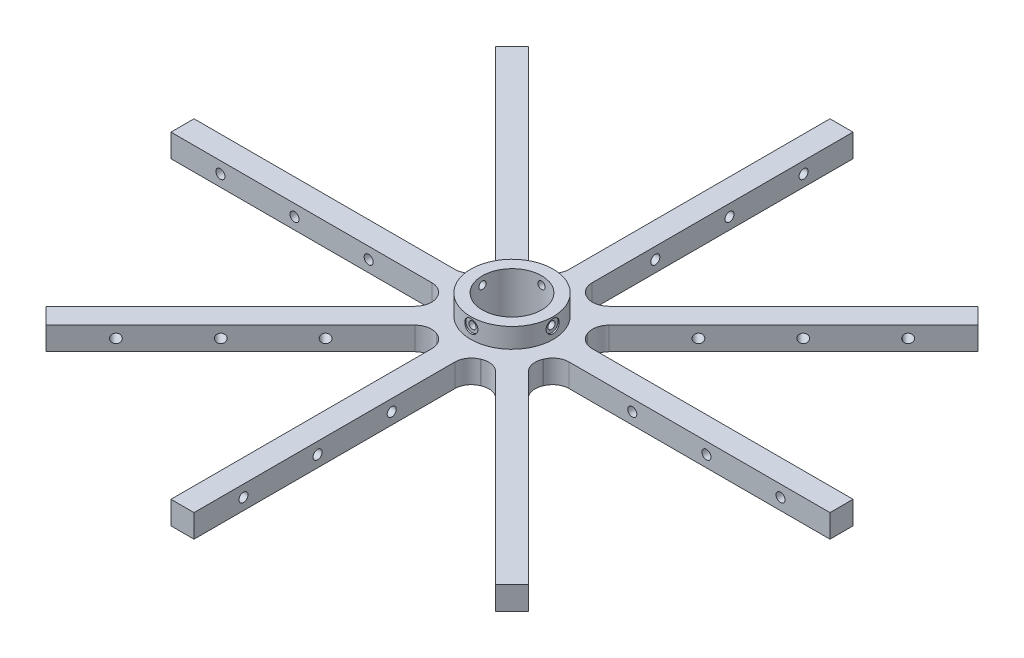
from build123d import *
from build123d.topology import SkipClean

# Parameters (mm, degrees)
SKETCH_3_R               = 25
SKETCH_3_R_2             = 18
EXTRUDE_4_DEPTH          = 7
SKETCH_4_W               = 176
SKETCH_4_H               = 14
EXTRUDE_5_DEPTH          = 7
SKETCH_5_R               = 2.75
CUT_EXTRUDE_1_DEPTH      = 14
PATTERN_CIRCULAR_1_COUNT = 8
EXTRUDE_START            = 12
SKETCH_6_R               = 25
SKETCH_6_R_2             = 18
EXTRUDE_6_DEPTH          = 12
SKETCH_7_R               = 2.2
CUT_EXTRUDE_2_DEPTH      = 43
CUT_EXTRUDE_START        = -24
SKETCH_8_R               = 4
CUT_EXTRUDE_4_DEPTH      = 43
PATTERN_CIRCULAR_2_COUNT = 4
SKETCH_10_R              = 35
SKETCH_10_R_2            = 25
EXTRUDE_7_DEPTH          = 14
FILLET_2_R               = 10


with BuildPart() as part:
    # 草图3 → 凸台-拉伸4 (new, symmetric)
    with BuildSketch(Plane(origin=(0, 0, 0), x_dir=(1, 0, 0), z_dir=(0, 1, 0))):
        with Locations(Location((0, 0, 0), (0, 0, 270))):
            Circle(SKETCH_3_R)
        with Locations(Location((0, 0, 0), (0, 0, 270))):
            Circle(SKETCH_3_R_2, mode=Mode.SUBTRACT)
    extrude(amount=EXTRUDE_4_DEPTH, both=True)

    # 草图4 → 凸台-拉伸5 (add, symmetric)
    with BuildSketch(Plane(origin=(0, 0, 0), x_dir=(1, 0, 0), z_dir=(0, 1, 0))):
        with Locations((112, 0)):
            Rectangle(SKETCH_4_W, SKETCH_4_H)
    extrude_5 = extrude(amount=EXTRUDE_5_DEPTH, both=True)

    # 草图5 → 切除-拉伸1 (cut)
    with BuildSketch(Plane.XY.offset(7)):
        with Locations((80, 0)):
            Circle(SKETCH_5_R)
        with Locations((125, 0)):
            Circle(SKETCH_5_R)
        with Locations((170, 0)):
            Circle(SKETCH_5_R)
    cut_extrude_1 = extrude(amount=-CUT_EXTRUDE_1_DEPTH, mode=Mode.SUBTRACT)

    # 阵列(圆周)1: 凸台-拉伸5, 切除-拉伸1 ×8 about axis
    pattern_circular_1_axis = Axis((0, 0, 0), (0, 1, 0))
    add([extrude_5.rotate(pattern_circular_1_axis, i * 360 / PATTERN_CIRCULAR_1_COUNT) for i in range(1, PATTERN_CIRCULAR_1_COUNT)])
    add([cut_extrude_1.rotate(pattern_circular_1_axis, i * 360 / PATTERN_CIRCULAR_1_COUNT) for i in range(1, PATTERN_CIRCULAR_1_COUNT)], mode=Mode.SUBTRACT)

    # 草图6 → 凸台-拉伸6 (add)
    with SkipClean():  # the faces are left unmerged after this step: merging them gives an invalid solid
        with BuildSketch(Plane(origin=(0, 7, 0), x_dir=(1, 0, 0), z_dir=(0, 1, 0)).offset(EXTRUDE_START)):
            with Locations(Location((0, 0, 0), (0, 0, 106.260204708))):
                Circle(SKETCH_6_R)
            with Locations(Location((0, 0, 0), (0, 0, 270))):
                Circle(SKETCH_6_R_2, mode=Mode.SUBTRACT)
        extrude(amount=-EXTRUDE_6_DEPTH)

    # 草图7 → 切除-拉伸2 (cut)
    with SkipClean():  # the faces are left unmerged after this step: merging them gives an invalid solid
        with BuildSketch(Plane.XY):
            with Locations(Location((0, 14, 0), (0, 0, 90))):
                Circle(SKETCH_7_R)
        cut_extrude_2 = extrude(amount=-CUT_EXTRUDE_2_DEPTH, mode=Mode.SUBTRACT)

    # 草图8 → 切除-拉伸4 (cut)
    with SkipClean():  # the faces are left unmerged after this step: merging them gives an invalid solid
        with BuildSketch(Plane.XY.offset(CUT_EXTRUDE_START)):
            with Locations((0, 14)):
                Circle(SKETCH_8_R)
        cut_extrude_4 = extrude(amount=-CUT_EXTRUDE_4_DEPTH, mode=Mode.SUBTRACT)

    # 阵列(圆周)2: 切除-拉伸2, 切除-拉伸4 ×4 about axis
    with SkipClean():  # the faces are left unmerged after this step: merging them gives an invalid solid
        pattern_circular_2_axis = Axis((0, 0, 0), (0, 1, 0))
        add([cut_extrude_2.rotate(pattern_circular_2_axis, i * 360 / PATTERN_CIRCULAR_2_COUNT) for i in range(1, PATTERN_CIRCULAR_2_COUNT)], mode=Mode.SUBTRACT)
        add([cut_extrude_4.rotate(pattern_circular_2_axis, i * 360 / PATTERN_CIRCULAR_2_COUNT) for i in range(1, PATTERN_CIRCULAR_2_COUNT)], mode=Mode.SUBTRACT)

    # 草图10 → 凸台-拉伸7 (add)
    with BuildSketch(Plane(origin=(0, 7, 0), x_dir=(1, 0, 0), z_dir=(0, 1, 0))):
        Circle(SKETCH_10_R)
        with Locations(Location((0, 0, 0), (0, 0, 270))):
            Circle(SKETCH_10_R_2, mode=Mode.SUBTRACT)
    extrude(amount=-EXTRUDE_7_DEPTH)

    # 圆角2
    fillet_2_edges = [part.edges().sort_by_distance(p)[0] for p in [
        (19.298963838, 0, -29.198458774),
        (34.292856399, 0, 7),
        (34.292856399, 0, -7),
        (19.298963838, 0, 29.198458774),
        (29.198458774, 0, 19.298963838),
        (-7, 0, 34.292856399),
        (7, 0, 34.292856399),
        (-29.198458774, 0, 19.298963838),
        (-19.298963838, 0, 29.198458774),
        (-34.292856399, 0, -7),
        (-34.292856399, 0, 7),
        (-19.298963838, 0, -29.198458774),
        (-29.198458774, 0, -19.298963838),
        (7, 0, -34.292856399),
        (-7, 0, -34.292856399),
        (29.198458774, 0, -19.298963838),
    ]]
    fillet(fillet_2_edges, radius=FILLET_2_R)


solid = part.part
